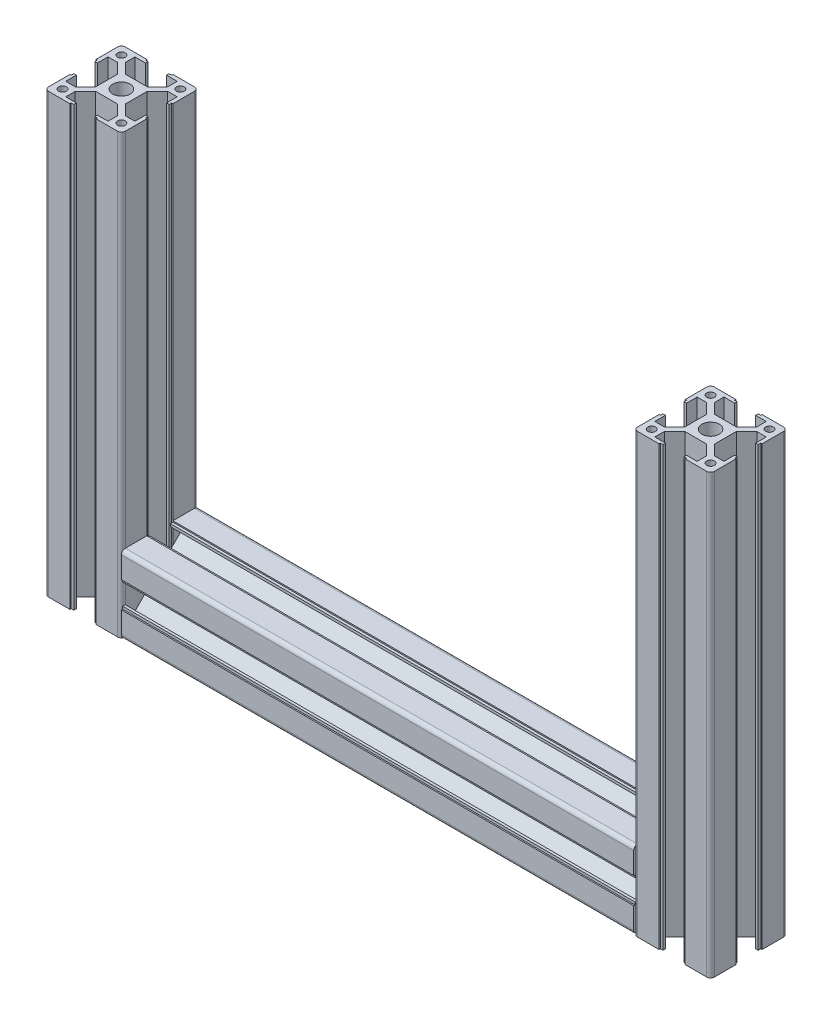
from build123d import *

# Parameters (mm, degrees)
SKETCH11_R                 = 3.4
SKETCH11_R_2               = 1.5
F_30X_30G_X_R1_5_1_DEPTH   = 171
SKETCH11_ON_SEGMENT_2_R    = 3.4
SKETCH11_ON_SEGMENT_2_R_2  = 1.5
F_30X_30G_X_R1_5_1_2_DEPTH = 171
SKETCH11_ON_SEGMENT_3_R    = 3.4
SKETCH11_ON_SEGMENT_3_R_2  = 1.5
F_30X_30G_X_R1_5_1_3_DEPTH = 232


with BuildPart() as part:
    # Sketch11 → 铝型材库 30X 30G X R1.5(1) (new body)
    with BuildSketch(Plane(origin=(-115, 78, 0), x_dir=(1, 0, 0), z_dir=(0, -1, 0))):
        with BuildLine():
            Line((-5.1, 15), (-5.1, 14.5))
            Line((-5.1, 14.5), (-4.1, 14.5))
            Line((-4.1, 14.5), (-4.1, 13.5))
            Line((-4.1, 13.5), (-8.25, 13.5))
            Line((-8.25, 13.5), (-8.25, 9.8))
            Line((-8.25, 9.8), (-4.25, 5.8))
            Line((-4.25, 5.8), (4.25, 5.8))
            Line((4.25, 5.8), (8.25, 9.8))
            Line((8.25, 9.8), (8.25, 13.5))
            Line((8.25, 13.5), (4.1, 13.5))
            Line((4.1, 13.5), (4.1, 14.5))
            Line((4.1, 14.5), (5.1, 14.5))
            Line((5.1, 14.5), (5.1, 15))
            Line((5.1, 15), (13.5, 15))
            ThreePointArc((13.5, 15), (14.560660172, 14.560660172), (15, 13.5))
            Line((15, 13.5), (15, 5.1))
            Line((15, 5.1), (14.5, 5.1))
            Line((14.5, 5.1), (14.5, 4.1))
            Line((14.5, 4.1), (13.5, 4.1))
            Line((13.5, 4.1), (13.5, 8.25))
            Line((13.5, 8.25), (9.8, 8.25))
            Line((9.8, 8.25), (5.8, 4.25))
            Line((5.8, 4.25), (5.8, -4.25))
            Line((5.8, -4.25), (9.8, -8.25))
            Line((9.8, -8.25), (13.5, -8.25))
            Line((13.5, -8.25), (13.5, -4.1))
            Line((13.5, -4.1), (14.5, -4.1))
            Line((14.5, -4.1), (14.5, -5.1))
            Line((14.5, -5.1), (15, -5.1))
            Line((15, -5.1), (15, -13.5))
            ThreePointArc((15, -13.5), (14.560660172, -14.560660172), (13.5, -15))
            Line((13.5, -15), (5.1, -15))
            Line((5.1, -15), (5.1, -14.5))
            Line((5.1, -14.5), (4.1, -14.5))
            Line((4.1, -14.5), (4.1, -13.5))
            Line((4.1, -13.5), (8.25, -13.5))
            Line((8.25, -13.5), (8.25, -9.8))
            Line((8.25, -9.8), (4.25, -5.8))
            Line((4.25, -5.8), (-4.25, -5.8))
            Line((-4.25, -5.8), (-8.25, -9.8))
            Line((-8.25, -9.8), (-8.25, -13.5))
            Line((-8.25, -13.5), (-4.1, -13.5))
            Line((-4.1, -13.5), (-4.1, -14.5))
            Line((-4.1, -14.5), (-5.1, -14.5))
            Line((-5.1, -14.5), (-5.1, -15))
            Line((-5.1, -15), (-13.5, -15))
            ThreePointArc((-13.5, -15), (-14.560660172, -14.560660172), (-15, -13.5))
            Line((-15, -13.5), (-15, -5.1))
            Line((-15, -5.1), (-14.5, -5.1))
            Line((-14.5, -5.1), (-14.5, -4.1))
            Line((-14.5, -4.1), (-13.5, -4.1))
            Line((-13.5, -4.1), (-13.5, -8.25))
            Line((-13.5, -8.25), (-9.8, -8.25))
            Line((-9.8, -8.25), (-5.8, -4.25))
            Line((-5.8, -4.25), (-5.8, 4.25))
            Line((-5.8, 4.25), (-9.8, 8.25))
            Line((-9.8, 8.25), (-13.5, 8.25))
            Line((-13.5, 8.25), (-13.5, 4.1))
            Line((-13.5, 4.1), (-14.5, 4.1))
            Line((-14.5, 4.1), (-14.5, 5.1))
            Line((-14.5, 5.1), (-15, 5.1))
            Line((-15, 5.1), (-15, 13.5))
            ThreePointArc((-15, 13.5), (-14.560660172, 14.560660172), (-13.5, 15))
            Line((-13.5, 15), (-5.1, 15))
        make_face()
        Circle(SKETCH11_R, mode=Mode.SUBTRACT)
        with Locations((-11.5, 11.5)):
            Circle(SKETCH11_R_2, mode=Mode.SUBTRACT)
        with Locations((11.5, 11.5)):
            Circle(SKETCH11_R_2, mode=Mode.SUBTRACT)
        with Locations((-11.5, -11.5)):
            Circle(SKETCH11_R_2, mode=Mode.SUBTRACT)
        with Locations((11.5, -11.5)):
            Circle(SKETCH11_R_2, mode=Mode.SUBTRACT)
    extrude(amount=F_30X_30G_X_R1_5_1_DEPTH)


with BuildPart() as body_2:
    # Sketch11 on segment 2 (carried to segment 2) → 30X 30G X R1.5_1 2 (new body)
    with BuildSketch(Plane(origin=(115, 78, 0), x_dir=(1, 0, 0), z_dir=(0, -1, 0))):
        with BuildLine():
            Line((-5.1, 15), (-5.1, 14.5))
            Line((-5.1, 14.5), (-4.1, 14.5))
            Line((-4.1, 14.5), (-4.1, 13.5))
            Line((-4.1, 13.5), (-8.25, 13.5))
            Line((-8.25, 13.5), (-8.25, 9.8))
            Line((-8.25, 9.8), (-4.25, 5.8))
            Line((-4.25, 5.8), (4.25, 5.8))
            Line((4.25, 5.8), (8.25, 9.8))
            Line((8.25, 9.8), (8.25, 13.5))
            Line((8.25, 13.5), (4.1, 13.5))
            Line((4.1, 13.5), (4.1, 14.5))
            Line((4.1, 14.5), (5.1, 14.5))
            Line((5.1, 14.5), (5.1, 15))
            Line((5.1, 15), (13.5, 15))
            ThreePointArc((13.5, 15), (14.560660172, 14.560660172), (15, 13.5))
            Line((15, 13.5), (15, 5.1))
            Line((15, 5.1), (14.5, 5.1))
            Line((14.5, 5.1), (14.5, 4.1))
            Line((14.5, 4.1), (13.5, 4.1))
            Line((13.5, 4.1), (13.5, 8.25))
            Line((13.5, 8.25), (9.8, 8.25))
            Line((9.8, 8.25), (5.8, 4.25))
            Line((5.8, 4.25), (5.8, -4.25))
            Line((5.8, -4.25), (9.8, -8.25))
            Line((9.8, -8.25), (13.5, -8.25))
            Line((13.5, -8.25), (13.5, -4.1))
            Line((13.5, -4.1), (14.5, -4.1))
            Line((14.5, -4.1), (14.5, -5.1))
            Line((14.5, -5.1), (15, -5.1))
            Line((15, -5.1), (15, -13.5))
            ThreePointArc((15, -13.5), (14.560660172, -14.560660172), (13.5, -15))
            Line((13.5, -15), (5.1, -15))
            Line((5.1, -15), (5.1, -14.5))
            Line((5.1, -14.5), (4.1, -14.5))
            Line((4.1, -14.5), (4.1, -13.5))
            Line((4.1, -13.5), (8.25, -13.5))
            Line((8.25, -13.5), (8.25, -9.8))
            Line((8.25, -9.8), (4.25, -5.8))
            Line((4.25, -5.8), (-4.25, -5.8))
            Line((-4.25, -5.8), (-8.25, -9.8))
            Line((-8.25, -9.8), (-8.25, -13.5))
            Line((-8.25, -13.5), (-4.1, -13.5))
            Line((-4.1, -13.5), (-4.1, -14.5))
            Line((-4.1, -14.5), (-5.1, -14.5))
            Line((-5.1, -14.5), (-5.1, -15))
            Line((-5.1, -15), (-13.5, -15))
            ThreePointArc((-13.5, -15), (-14.560660172, -14.560660172), (-15, -13.5))
            Line((-15, -13.5), (-15, -5.1))
            Line((-15, -5.1), (-14.5, -5.1))
            Line((-14.5, -5.1), (-14.5, -4.1))
            Line((-14.5, -4.1), (-13.5, -4.1))
            Line((-13.5, -4.1), (-13.5, -8.25))
            Line((-13.5, -8.25), (-9.8, -8.25))
            Line((-9.8, -8.25), (-5.8, -4.25))
            Line((-5.8, -4.25), (-5.8, 4.25))
            Line((-5.8, 4.25), (-9.8, 8.25))
            Line((-9.8, 8.25), (-13.5, 8.25))
            Line((-13.5, 8.25), (-13.5, 4.1))
            Line((-13.5, 4.1), (-14.5, 4.1))
            Line((-14.5, 4.1), (-14.5, 5.1))
            Line((-14.5, 5.1), (-15, 5.1))
            Line((-15, 5.1), (-15, 13.5))
            ThreePointArc((-15, 13.5), (-14.560660172, 14.560660172), (-13.5, 15))
            Line((-13.5, 15), (-5.1, 15))
        make_face()
        Circle(SKETCH11_ON_SEGMENT_2_R, mode=Mode.SUBTRACT)
        with Locations((-11.5, 11.5)):
            Circle(SKETCH11_ON_SEGMENT_2_R_2, mode=Mode.SUBTRACT)
        with Locations((11.5, 11.5)):
            Circle(SKETCH11_ON_SEGMENT_2_R_2, mode=Mode.SUBTRACT)
        with Locations((-11.5, -11.5)):
            Circle(SKETCH11_ON_SEGMENT_2_R_2, mode=Mode.SUBTRACT)
        with Locations((11.5, -11.5)):
            Circle(SKETCH11_ON_SEGMENT_2_R_2, mode=Mode.SUBTRACT)
    extrude(amount=F_30X_30G_X_R1_5_1_2_DEPTH)


with BuildPart() as body_3:
    # Sketch11 on segment 3 (carried to segment 3) → 30X 30G X R1.5_1 3 (new body)
    with BuildSketch(Plane(origin=(-116, -78, 0), x_dir=(0, 1, 0), z_dir=(1, 0, 0))):
        with BuildLine():
            Line((-5.1, 15), (-5.1, 14.5))
            Line((-5.1, 14.5), (-4.1, 14.5))
            Line((-4.1, 14.5), (-4.1, 13.5))
            Line((-4.1, 13.5), (-8.25, 13.5))
            Line((-8.25, 13.5), (-8.25, 9.8))
            Line((-8.25, 9.8), (-4.25, 5.8))
            Line((-4.25, 5.8), (4.25, 5.8))
            Line((4.25, 5.8), (8.25, 9.8))
            Line((8.25, 9.8), (8.25, 13.5))
            Line((8.25, 13.5), (4.1, 13.5))
            Line((4.1, 13.5), (4.1, 14.5))
            Line((4.1, 14.5), (5.1, 14.5))
            Line((5.1, 14.5), (5.1, 15))
            Line((5.1, 15), (13.5, 15))
            ThreePointArc((13.5, 15), (14.560660172, 14.560660172), (15, 13.5))
            Line((15, 13.5), (15, 5.1))
            Line((15, 5.1), (14.5, 5.1))
            Line((14.5, 5.1), (14.5, 4.1))
            Line((14.5, 4.1), (13.5, 4.1))
            Line((13.5, 4.1), (13.5, 8.25))
            Line((13.5, 8.25), (9.8, 8.25))
            Line((9.8, 8.25), (5.8, 4.25))
            Line((5.8, 4.25), (5.8, -4.25))
            Line((5.8, -4.25), (9.8, -8.25))
            Line((9.8, -8.25), (13.5, -8.25))
            Line((13.5, -8.25), (13.5, -4.1))
            Line((13.5, -4.1), (14.5, -4.1))
            Line((14.5, -4.1), (14.5, -5.1))
            Line((14.5, -5.1), (15, -5.1))
            Line((15, -5.1), (15, -13.5))
            ThreePointArc((15, -13.5), (14.560660172, -14.560660172), (13.5, -15))
            Line((13.5, -15), (5.1, -15))
            Line((5.1, -15), (5.1, -14.5))
            Line((5.1, -14.5), (4.1, -14.5))
            Line((4.1, -14.5), (4.1, -13.5))
            Line((4.1, -13.5), (8.25, -13.5))
            Line((8.25, -13.5), (8.25, -9.8))
            Line((8.25, -9.8), (4.25, -5.8))
            Line((4.25, -5.8), (-4.25, -5.8))
            Line((-4.25, -5.8), (-8.25, -9.8))
            Line((-8.25, -9.8), (-8.25, -13.5))
            Line((-8.25, -13.5), (-4.1, -13.5))
            Line((-4.1, -13.5), (-4.1, -14.5))
            Line((-4.1, -14.5), (-5.1, -14.5))
            Line((-5.1, -14.5), (-5.1, -15))
            Line((-5.1, -15), (-13.5, -15))
            ThreePointArc((-13.5, -15), (-14.560660172, -14.560660172), (-15, -13.5))
            Line((-15, -13.5), (-15, -5.1))
            Line((-15, -5.1), (-14.5, -5.1))
            Line((-14.5, -5.1), (-14.5, -4.1))
            Line((-14.5, -4.1), (-13.5, -4.1))
            Line((-13.5, -4.1), (-13.5, -8.25))
            Line((-13.5, -8.25), (-9.8, -8.25))
            Line((-9.8, -8.25), (-5.8, -4.25))
            Line((-5.8, -4.25), (-5.8, 4.25))
            Line((-5.8, 4.25), (-9.8, 8.25))
            Line((-9.8, 8.25), (-13.5, 8.25))
            Line((-13.5, 8.25), (-13.5, 4.1))
            Line((-13.5, 4.1), (-14.5, 4.1))
            Line((-14.5, 4.1), (-14.5, 5.1))
            Line((-14.5, 5.1), (-15, 5.1))
            Line((-15, 5.1), (-15, 13.5))
            ThreePointArc((-15, 13.5), (-14.560660172, 14.560660172), (-13.5, 15))
            Line((-13.5, 15), (-5.1, 15))
        make_face()
        Circle(SKETCH11_ON_SEGMENT_3_R, mode=Mode.SUBTRACT)
        with Locations((-11.5, 11.5)):
            Circle(SKETCH11_ON_SEGMENT_3_R_2, mode=Mode.SUBTRACT)
        with Locations((11.5, 11.5)):
            Circle(SKETCH11_ON_SEGMENT_3_R_2, mode=Mode.SUBTRACT)
        with Locations((-11.5, -11.5)):
            Circle(SKETCH11_ON_SEGMENT_3_R_2, mode=Mode.SUBTRACT)
        with Locations((11.5, -11.5)):
            Circle(SKETCH11_ON_SEGMENT_3_R_2, mode=Mode.SUBTRACT)
    extrude(amount=F_30X_30G_X_R1_5_1_3_DEPTH)

    # 30X 30G X R1.5_1 3 end butt 1
    split(bisect_by=Plane(origin=(-100, -78, 0), x_dir=(0, 1, 0), z_dir=(1, 0, 0)), keep=Keep.TOP)

    # 30X 30G X R1.5_1 3 end butt 2
    split(bisect_by=Plane(origin=(100, -78, 0), x_dir=(0, -1, 0), z_dir=(-1, 0, 0)), keep=Keep.TOP)


solid = Compound([part.part, body_2.part, body_3.part])
